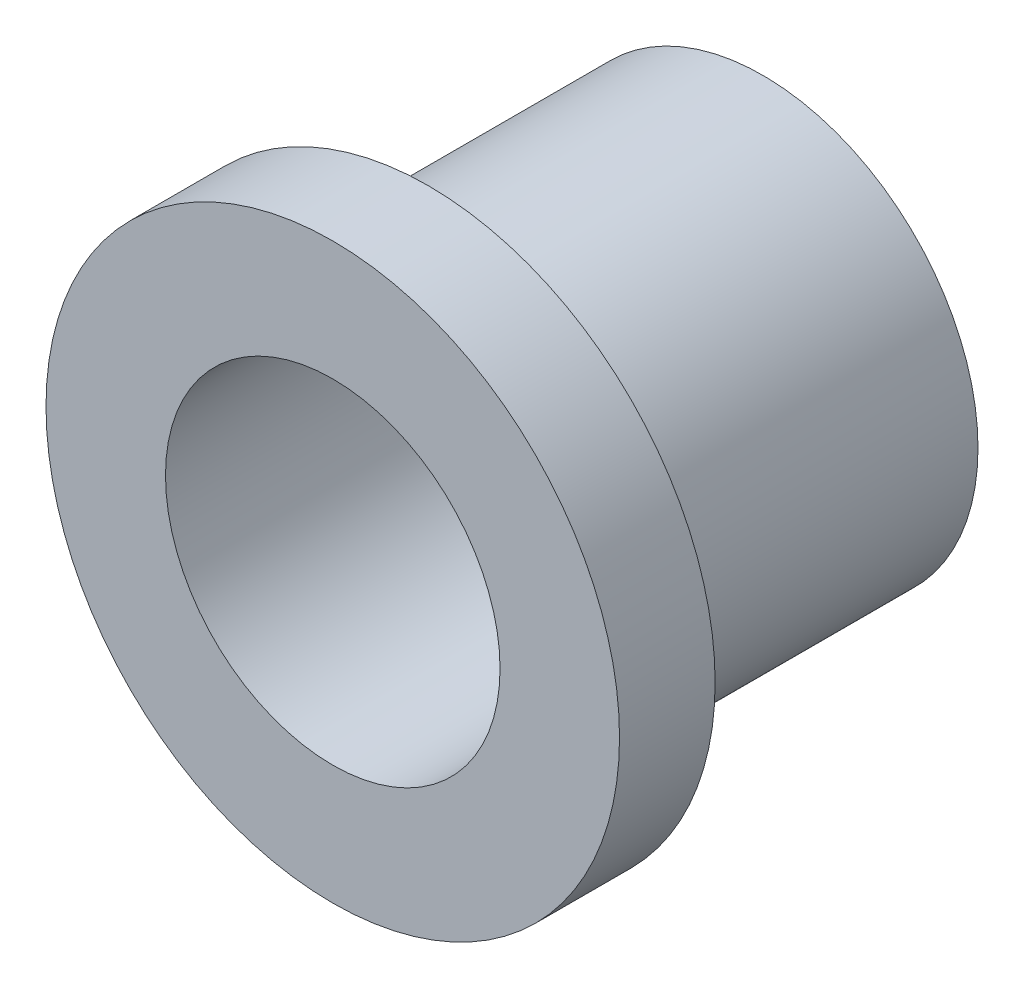
from build123d import *

# Parameters (mm, degrees)
SKETCH_1_R      = 6
SKETCH_1_R_2    = 3.5
EXTRUDE_1_DEPTH = 1
EXTRUDE_START   = -8
SKETCH_2_R      = 4.5
SKETCH_2_R_2    = 3.5
EXTRUDE_2_DEPTH = 8


with BuildPart() as part:
    # 草图1 → 凸台-拉伸1 (new, symmetric)
    with BuildSketch(Plane.XY):
        Circle(SKETCH_1_R)
        Circle(SKETCH_1_R_2, mode=Mode.SUBTRACT)
    extrude(amount=EXTRUDE_1_DEPTH, both=True)

    # 草图2 → 凸台-拉伸2 (add)
    with BuildSketch(Plane.XY.offset(EXTRUDE_START)):
        Circle(SKETCH_2_R)
        Circle(SKETCH_2_R_2, mode=Mode.SUBTRACT)
    extrude(amount=EXTRUDE_2_DEPTH)


solid = part.part
